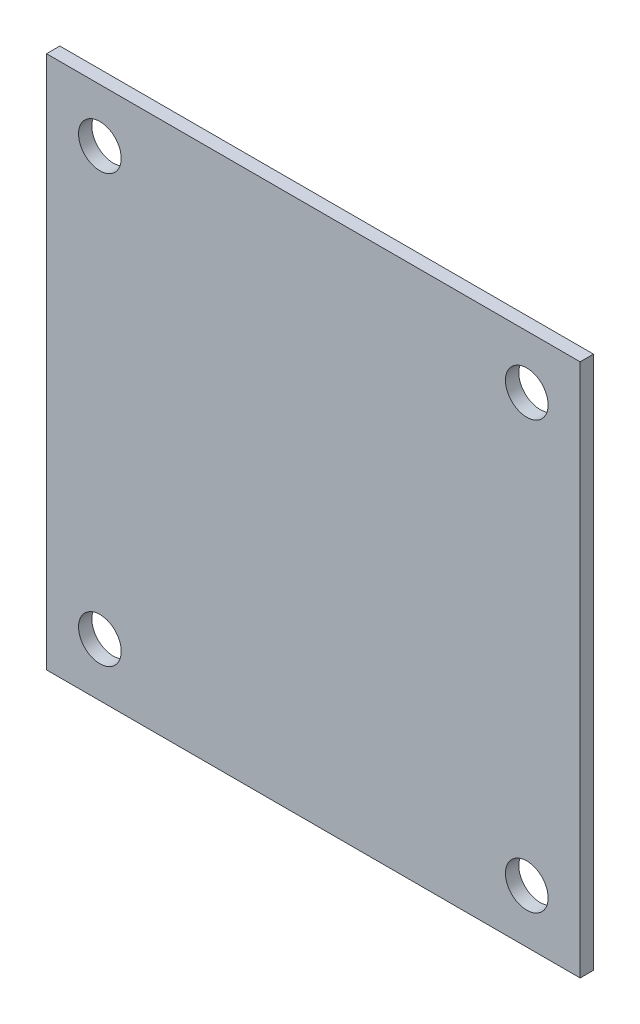
SolidWorks part; units mm, degrees
ref_plane "Front Plane" through (0, 0, 0) normal (0, 0, 1) x (1, 0, 0)
ref_plane "Top Plane" through (0, 0, 0) normal (0, 1, 0) x (1, 0, 0)
ref_plane "Right Plane" through (0, 0, 0) normal (1, 0, 0) x (0, 0, -1)
other "Configuration Table"
sketch "Sketch1" plane through (0, 0, 0) normal (0, 0, 1) x (1, 0, 0)
  line L1 (-200, 200) -> (200, 200)
  line L2 (-200, 200) -> (-200, -200)
  line L3 (-200, -200) -> (200, -200)
  line L4 (200, 200) -> (200, -200)
  line L5 (-200, 200) -> (200, -200) construction
  line L6 (-200, -200) -> (200, 200) construction
  line L7 (-160, 160) -> (160, 160) construction
  line L8 (-160, 160) -> (-160, -160) construction
  line L9 (-160, -160) -> (160, -160) construction
  line L10 (160, 160) -> (160, -160) construction
  line L11 (-160, 160) -> (160, -160) construction
  line L12 (-160, -160) -> (160, 160) construction
  circle A0 centre (-160, 160) radius 16
  circle A1 centre (160, 160) radius 16
  circle A2 centre (160, -160) radius 16
  circle A3 centre (-160, -160) radius 16
  point P0 (0, 0)
  point P6 (0, 0)
  dimension "D4" = 32
  dimension "D1" = 400
  dimension "D2" = 320
  dimension "400" = 400
  dimension "D3" = 320
extrude "Boss-Extrude1" add sketch "Sketch1" along normal blind 10
